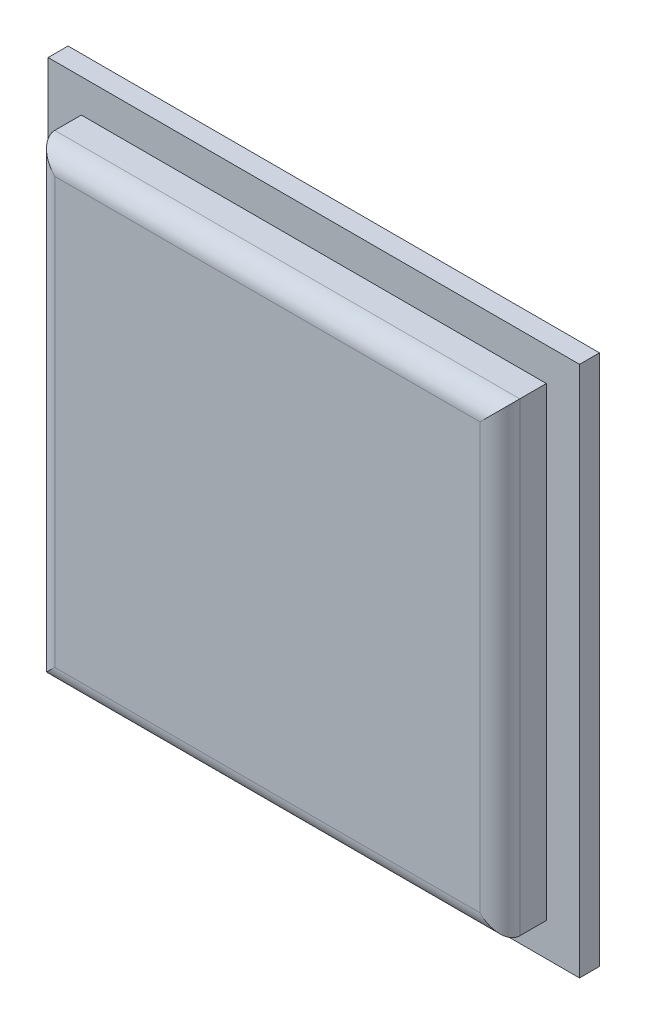
SolidWorks part; units mm, degrees
ref_plane "Front Plane" through (0, 0, 0) normal (0, 0, 1) x (1, 0, 0)
ref_plane "Top Plane" through (0, 0, 0) normal (0, 1, 0) x (1, 0, 0)
ref_plane "Right Plane" through (0, 0, 0) normal (1, 0, 0) x (0, 0, -1)
other "Configuration Table"
sketch "Sketch1" plane through (0, 0, 0) normal (0, 0, 1) x (1, 0, 0)
  line L1 (-40, 40) -> (40, 40)
  line L2 (-40, 40) -> (-40, -40)
  line L3 (-40, -40) -> (40, -40)
  line L4 (40, 40) -> (40, -40)
  line L5 (-40, 40) -> (40, -40) construction
  line L6 (-40, -40) -> (40, 40) construction
  point P0 (0, 0)
  dimension "D1" = 80
  dimension "D2" = 80
extrude "Boss-Extrude1" add sketch "Sketch1" along normal blind 3
sketch "Sketch2" plane through (0, 0, 3) normal (0, 0, 1) x (1, 0, 0)
  line L1 (-35, 35) -> (35, 35)
  line L2 (-35, 35) -> (-35, -35)
  line L3 (-35, -35) -> (35, -35)
  line L4 (35, 35) -> (35, -35)
  line L5 (-35, 35) -> (35, -35) construction
  line L6 (-35, -35) -> (35, 35) construction
  point P0 (0, 0)
  dimension "D1" = 70
  dimension "D2" = 70
extrude "Boss-Extrude2" add sketch "Sketch2" along normal blind 7
fillet "Fillet1" radius 3 4 edges at (0, -35, 10) (-35, 0, 10) (0, 35, 10) (35, 0, 10)
